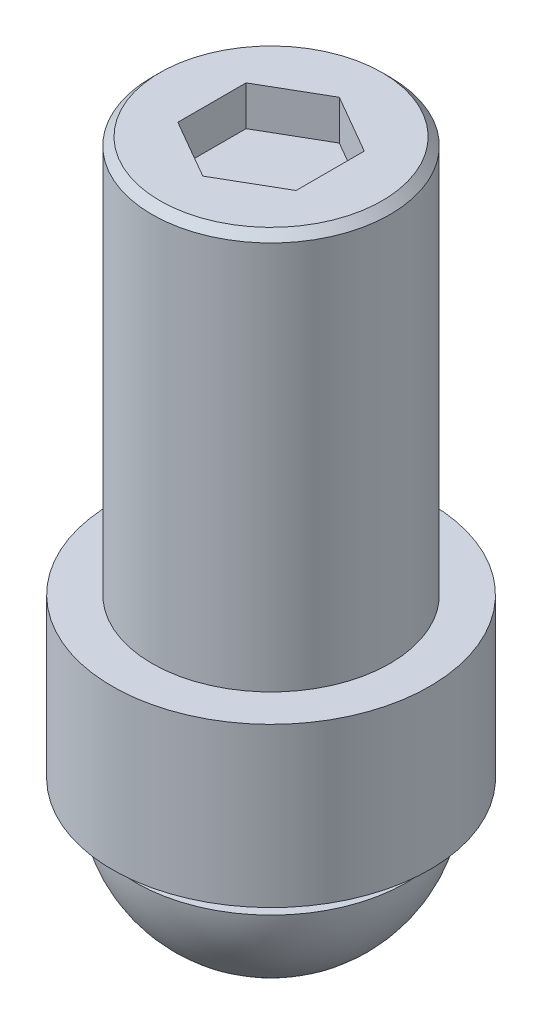
from build123d import *

# Parameters (mm, degrees)
SKETCH1_R           = 1.5
BOSS_EXTRUDE1_DEPTH = 5
SKETCH2_R           = 2
BOSS_EXTRUDE2_DEPTH = 2
CUT_EXTRUDE1_DEPTH  = 0.5
CHAMFER1_SIZE       = 0.1


with BuildPart() as part:
    # Sketch1 → Boss-Extrude1 (new body)
    with BuildSketch(Plane(origin=(0, 0, 0), x_dir=(1, 0, 0), z_dir=(0, 1, 0))):
        with Locations(Location((0, 0, 0), (0, 0, 270))):
            Circle(SKETCH1_R)
    extrude(amount=BOSS_EXTRUDE1_DEPTH)

    # Sketch2 → Boss-Extrude2 (add)
    with BuildSketch(Plane.XZ):
        with Locations(Location((0, 0, 0), (0, 0, 270))):
            Circle(SKETCH2_R)
    extrude(amount=BOSS_EXTRUDE2_DEPTH)

    # Sketch3 → Revolve1 (revolve)
    with BuildSketch(Plane.XY):
        with BuildLine():
            Line((0, -2), (0, -3.798690772))
            ThreePointArc((0, -3.798690772), (1.135010023, -3.368611599), (1.7, -2.294366668))
            Line((1.7, -2.294366668), (1.376675655, -2.294366668))
            Line((1.376675655, -2.294366668), (1.376675655, -2))
            Line((1.376675655, -2), (0, -2))
        make_face()
    revolve(axis=Axis((0, -2, 0), (0, -1, 0)))

    # Sketch4 → Cut-Extrude1 (cut)
    with BuildSketch(Plane(origin=(0, 5, 0), x_dir=(1, 0, 0), z_dir=(0, 1, 0))):
        Polygon((0, 0.860152501), (-0.744913917, 0.430076251), (-0.744913917, -0.430076251), (0, -0.860152501), (0.744913917, -0.430076251), (0.744913917, 0.430076251), align=None)
    extrude(amount=-CUT_EXTRUDE1_DEPTH, mode=Mode.SUBTRACT)

    # Chamfer1
    chamfer1_edges = [part.edges().sort_by_distance(p)[0] for p in [
        (0, 5, -1.5),
    ]]
    chamfer(chamfer1_edges, length=CHAMFER1_SIZE)


solid = part.part
